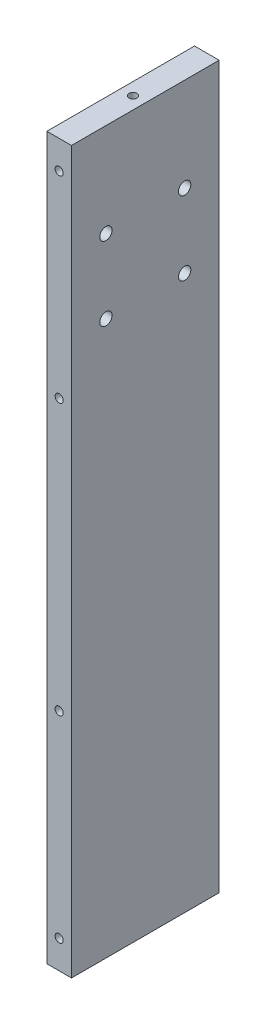
SolidWorks part; units mm, degrees
ref_plane "Front Plane" through (0, 0, 0) normal (0, 0, 1) x (1, 0, 0)
ref_plane "Top Plane" through (0, 0, 0) normal (0, 1, 0) x (1, 0, 0)
ref_plane "Right Plane" through (0, 0, 0) normal (1, 0, 0) x (0, 0, -1)
sketch "Sketch1" plane through (0, 0, 0) normal (0, 0, 1) x (1, 0, 0)
  line L1 (5, 146.5) -> (-5, 146.5)
  line L2 (5, 146.5) -> (5, -146.5)
  line L3 (5, -146.5) -> (-5, -146.5)
  line L4 (-5, 146.5) -> (-5, -146.5)
  line L5 (5, 146.5) -> (-5, -146.5) construction
  line L6 (5, -146.5) -> (-5, 146.5) construction
  point P0 (0, 0)
  dimension "D1" = 10
  dimension "D2" = 293
extrude "Boss-Extrude1" add sketch "Sketch1" along normal mid plane 60
hole_wizard "M4 Tapped Hole1" positions "Sketch5" profile "Sketch4" tap size "M4" standard "Gb"
sketch "Sketch5" plane through (0, 0, 30) normal (0, 0, 1) x (1, 0, 0)
  point P0 (0, 135)
  point P5 (0, -135)
  point P7 (0, 55)
  point P9 (0, -55)
  dimension "D1" = 110
  dimension "D2" = 55
  dimension "D3" = 80
  dimension "D4" = 80
sketch "Sketch4" plane through (0, 135, 30) normal (1, 0, 0) x (0, -1, 0)
  line L0 (0, 0) -> (0, 12.4914)
  line L1 (0, 12.4914) -> (1.65, 11.5)
  line L2 (1.65, 11.5) -> (1.65, 0)
  line L5 (1.65, 0) -> (0, 0)
  line L10 (0, 12.4914) -> (-1.65, 11.5) construction
  line L11 (0, -6.35) -> (0, 107.95) construction
  dimension "螺纹孔钻头直径" = 3.3
  dimension "螺纹孔钻头深度" = 11.5
  dimension "导头角度" = 118
cosmetic thread "Cosmetic thread 1" parameters "D1"=8, "D2"=4
cosmetic thread "Cosmetic thread 2" parameters "D1"=8, "D2"=4
cosmetic thread "Cosmetic thread 3" parameters "D1"=8, "D2"=4
cosmetic thread "Cosmetic thread 4" parameters "D1"=8, "D2"=4
hole_wizard "M4 Tapped Hole2" positions "Sketch7" profile "Sketch6" tap size "M4" standard "Gb"
sketch "Sketch7" plane through (0, -146.5, 0) normal (0, -1, 0) x (-1, 0, 0)
  point P0 (0, 0)
sketch "Sketch6" plane through (0, -146.5, 0) normal (1, 0, 0) x (0, 0, -1)
  line L0 (0, 0) -> (0, 12.4914)
  line L1 (0, 12.4914) -> (1.65, 11.5)
  line L2 (1.65, 11.5) -> (1.65, 0)
  line L5 (1.65, 0) -> (0, 0)
  line L10 (0, 12.4914) -> (-1.65, 11.5) construction
  line L11 (0, -6.35) -> (0, 107.95) construction
  dimension "螺纹孔钻头直径" = 3.3
  dimension "螺纹孔钻头深度" = 11.5
  dimension "导头角度" = 118
cosmetic thread "Cosmetic thread 5" parameters "D1"=8, "D2"=4
mirror "Mirror1" about plane through (0, 0, 0) normal (0, 1, 0) of "M4 Tapped Hole2"
hole_wizard "M6 Tapped Hole1" positions "Sketch9" profile "Sketch8" tap size "M6" standard "Gb" end condition through all
sketch "Sketch9" plane through (5, 0, 0) normal (1, 0, 0) x (0, 0, -1)
  line L0 (-30, -146.5) -> (-30, 146.5) construction
  line L1 (-30, 146.5) -> (30, 146.5) construction
  point P0 (-16, 78.5)
  point P3 (16, 78.5)
  point P6 (16, 108.5)
  point P9 (-16, 108.5)
  dimension "D1" = 14
  dimension "D2" = 32
  dimension "D3" = 38
  dimension "D4" = 30
cosmetic thread "Cosmetic thread 8" parameters "D2"=6
cosmetic thread "Cosmetic thread 9" parameters "D2"=6
cosmetic thread "Cosmetic thread 12" parameters "D2"=6
cosmetic thread "Cosmetic thread 13" parameters "D2"=6
sketch "Sketch8" plane through (5, 78.5, 16) normal (0, 1, 0) x (0, 0, -1)
  line L0 (0, 0) -> (0, 10)
  line L1 (0, 10) -> (2.5, 10)
  line L2 (2.5, 10) -> (2.5, 0)
  line L5 (2.5, 0) -> (0, 0)
  line L11 (0, -6.35) -> (0, 107.95) construction
  dimension "通孔螺纹孔钻头直径" = 5
  dimension "通孔螺纹孔钻头深度" = 10
mirror "Mirror2" about plane through (0, 0, 0) normal (0, 0, 1) of "M4 Tapped Hole1"
